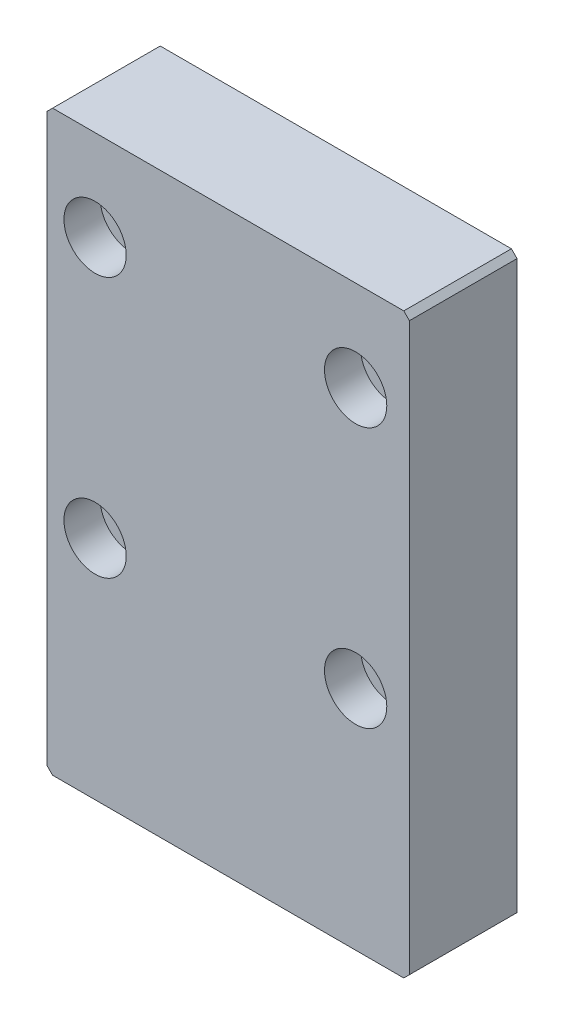
from build123d import *

# Parameters (mm, degrees)
SKETCH_15_W                  = 44
SKETCH_15_H                  = 120
EXTRUDE_1_DEPTH              = 19
HOLE_WIZARD_M4_2_D           = 3.3
HOLE_WIZARD_M4_2_DEPTH       = 11.5
HOLE_WIZARD_M4_2_TIP         = 0.991420021
SKETCH_21_W                  = 44
SKETCH_21_H                  = 18
CUT_EXTRUDE_4_DEPTH          = 19
HOLE_WIZARD_M4_1_D           = 3.3
HOLE_WIZARD_M4_1_DEPTH       = 10.1
HOLE_WIZARD_M4_1_TIP         = 0.991420021
CHAMFER_1_SIZE               = 1
SKETCH_24_W                  = 13.771291576
SKETCH_24_H                  = 102
SKETCH_24_W_2                = 13.032581782
EXTRUDE_2_DEPTH              = 19
HOLE_WIZARD_M6_1_D           = 6.6
HOLE_WIZARD_M6_1_CBORE_D     = 11
HOLE_WIZARD_M6_1_CBORE_DEPTH = 6.4
CHAMFER_2_SIZE               = 1


with BuildPart() as part:
    # 草图15 → 凸台-拉伸1 (new body)
    with BuildSketch(Plane.XY):
        with Locations((3.072247365, -30.72304468)):
            Rectangle(SKETCH_15_W, SKETCH_15_H)
    extrude(amount=EXTRUDE_1_DEPTH)

    # M4 螺纹孔2
    with Locations(Plane(origin=(0, 0, 0), x_dir=(-1, 0, 0), z_dir=(0, 0, -1))):
        with Locations((-3.072247365, 2.27695532), (-3.072247365, -26.72304468), (-3.072247365, -65.72304468)):
            Hole(HOLE_WIZARD_M4_2_D / 2, depth=HOLE_WIZARD_M4_2_DEPTH)
            with Locations((0, 0, -(HOLE_WIZARD_M4_2_DEPTH + HOLE_WIZARD_M4_2_TIP / 2))):  # 118° drill point
                Cone(0, HOLE_WIZARD_M4_2_D / 2, HOLE_WIZARD_M4_2_TIP, mode=Mode.SUBTRACT)

    # 草图21 → 切除-拉伸4 (cut)
    with BuildSketch(Plane.XY.offset(19)):
        with Locations((3.072247365, 20.27695532)):
            Rectangle(SKETCH_21_W, SKETCH_21_H)
    extrude(amount=-CUT_EXTRUDE_4_DEPTH, mode=Mode.SUBTRACT)

    # M4 螺纹孔1
    with Locations(Plane(origin=(0, 0, 0), x_dir=(-1, 0, 0), z_dir=(0, 0, -1))):
        with Locations((-13.072247365, 7.27695532), (6.927752635, 7.27695532)):
            Hole(HOLE_WIZARD_M4_1_D / 2, depth=HOLE_WIZARD_M4_1_DEPTH)
            with Locations((0, 0, -(HOLE_WIZARD_M4_1_DEPTH + HOLE_WIZARD_M4_1_TIP / 2))):  # 118° drill point
                Cone(0, HOLE_WIZARD_M4_1_D / 2, HOLE_WIZARD_M4_1_TIP, mode=Mode.SUBTRACT)

    # 倒角1
    chamfer_1_edges = [part.edges().sort_by_distance(p)[0] for p in [
        (-18.927752635, 11.27695532, 9.5),
        (25.072247365, 11.27695532, 9.5),
        (25.072247365, -90.72304468, 9.5),
        (-18.927752635, -90.72304468, 9.5),
    ]]
    chamfer(chamfer_1_edges, length=CHAMFER_1_SIZE)

    # 草图24 → 凸台-拉伸2 (add)
    with BuildSketch(Plane.XY.offset(19)):
        with Locations((-22.042106847, -39.72304468)):
            Rectangle(SKETCH_24_W, SKETCH_24_H)
        with Locations((28.555956474, -39.72304468)):
            Rectangle(SKETCH_24_W_2, SKETCH_24_H)
    extrude(amount=-EXTRUDE_2_DEPTH)

    # M6 六角凹头螺钉的柱形沉头孔1 (through all)
    with Locations(Plane.XY.offset(19)):
        with Locations((-20.427752635, -4.72304468), (25.572247365, -4.72304468), (25.572247365, -50.70304438), (-20.427752635, -50.72304468)):
            CounterBoreHole(HOLE_WIZARD_M6_1_D / 2, HOLE_WIZARD_M6_1_CBORE_D / 2, HOLE_WIZARD_M6_1_CBORE_DEPTH)

    # 倒角2
    chamfer_2_edges = [part.edges().sort_by_distance(p)[0] for p in [
        (35.072247365, -90.72304468, 9.5),
        (35.072247365, 11.27695532, 9.5),
        (-28.927752635, -90.72304468, 9.5),
        (-28.927752635, 11.27695532, 9.5),
    ]]
    chamfer(chamfer_2_edges, length=CHAMFER_2_SIZE)


solid = part.part
